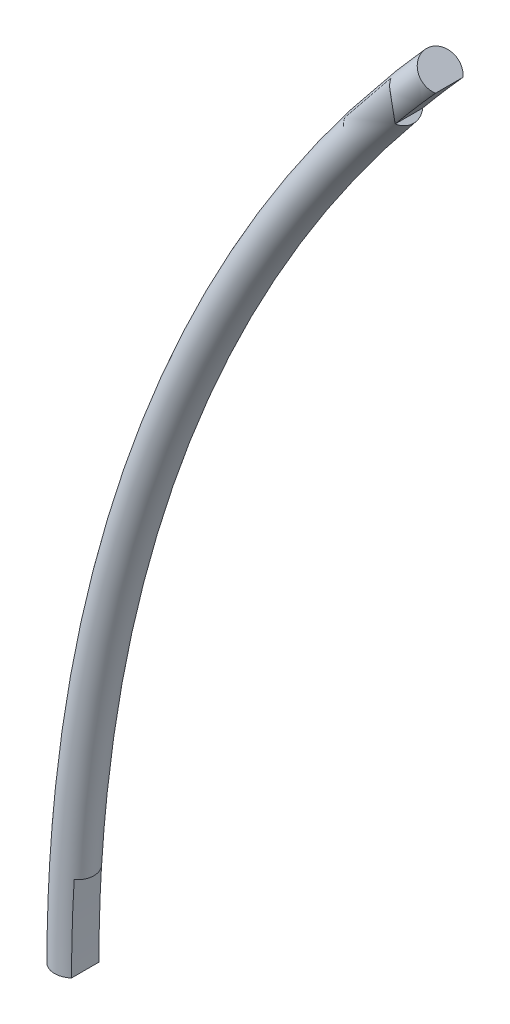
SolidWorks part; units mm, degrees
ref_plane "Front Plane" through (0, 0, 0) normal (0, 0, 1) x (1, 0, 0)
ref_plane "Top Plane" through (0, 0, 0) normal (0, 1, 0) x (1, 0, 0)
ref_plane "Right Plane" through (0, 0, 0) normal (1, 0, 0) x (0, 0, -1)
sketch "Sketch1" plane through (0, 0, 0) normal (0, 0, 1) x (1, 0, 0)
  line L0 (0, 0) -> (-121.3358, 0) construction
  line L1 (0, 0) -> (-83.0487, 74.7774) construction
  arc A0 (-173.1527, 155.9074) -> (-233, 0) centre (0, 0) ccw
  dimension "D1" = 42
  dimension "D2" = 233
sweep "Sweep1" add path "Sketch1" circular profile diameter 6 parameters "D3"=6
sketch "Sketch6" plane through (0, 0, 0) normal (0, 0, 1) x (1, 0, 0)
  line L0 (0, 0) -> (-231, 0)
  line L1 (0, 0) -> (-230.5691, 14.1022)
  line L2 (0, 0) -> (-178.2453, 146.9341)
  line L3 (0, 0) -> (-171.6665, 154.5692)
  line L4 (-170.9233, 153.9) -> (-175.3822, 157.9148) construction
  arc A0 (-171.6665, 154.5692) -> (-178.2453, 146.9341) centre (0, 0) ccw
  arc A1 (-230.5691, 14.1022) -> (-231, 0) centre (0, 0) ccw
  dimension "D1" = 462
  dimension "D2" = 3.5
  dimension "D3" = 36
extrude "Cut-Extrude1" cut sketch "Sketch6" against normal mid plane 50 contours L1 A1 L0 | L3 A0 L2
